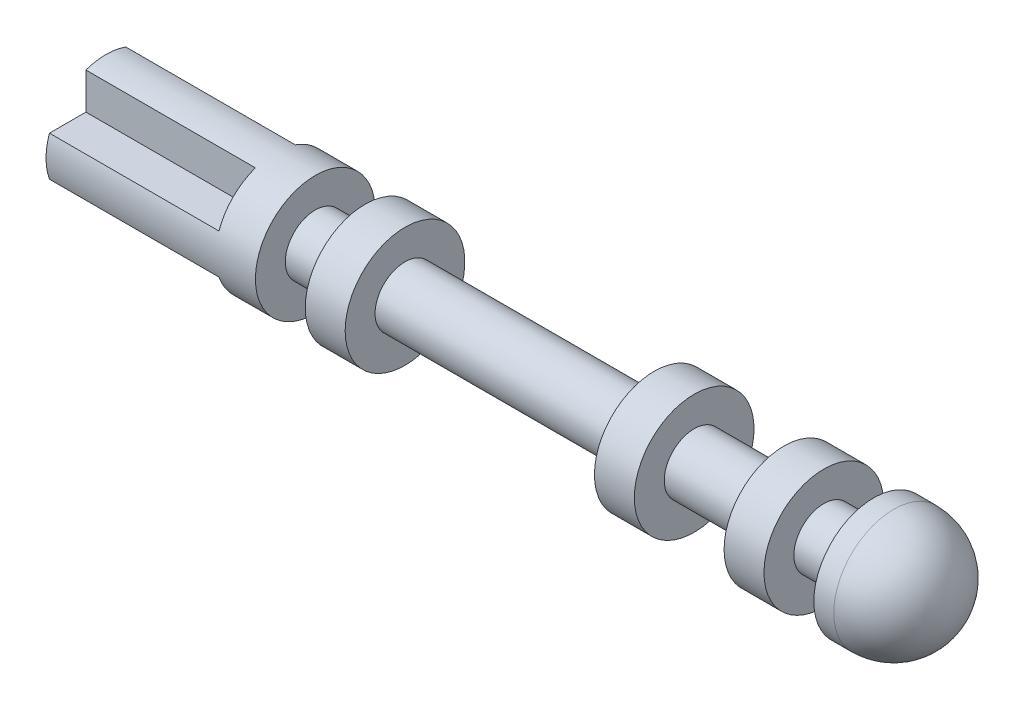
SolidWorks part; units mm, degrees
ref_plane "Front Plane" through (0, 0, 0) normal (0, 0, 1) x (1, 0, 0)
ref_plane "Top Plane" through (0, 0, 0) normal (0, 1, 0) x (1, 0, 0)
ref_plane "Right Plane" through (0, 0, 0) normal (1, 0, 0) x (0, 0, -1)
sketch "Sketch1" plane through (0, 0, 0) normal (0, 0, 1) x (1, 0, 0)
  line L0 (0, 0) -> (141.224, 0) construction
  line L1 (0, 0) -> (0, 3)
  line L2 (0, 3) -> (10.5, 3)
  line L3 (10.5, 3) -> (10.5, 1.5)
  line L4 (10.5, 1.5) -> (13, 1.5)
  line L5 (13, 1.5) -> (13, 3)
  line L6 (13, 3) -> (15, 3)
  line L7 (15, 3) -> (15, 1.5)
  line L8 (15, 1.5) -> (27.5, 1.5)
  line L9 (27.5, 1.5) -> (27.5, 3)
  line L10 (27.5, 3) -> (29.5, 3)
  line L11 (29.5, 3) -> (29.5, 1.5)
  line L12 (29.5, 1.5) -> (34, 1.5)
  line L13 (34, 1.5) -> (34, 3)
  line L14 (34, 3) -> (36, 3)
  line L15 (36, 3) -> (36, 1.5)
  line L16 (36, 1.5) -> (38.5, 1.5)
  line L17 (38.5, 1.5) -> (38.5, 3)
  line L18 (38.5, 3) -> (39.5, 3)
  line L19 (0, 0) -> (42.5, 0)
  arc A0 (39.5, 3) -> (42.5, 0) centre (39.5, 0) cw
  dimension "D5" = 3
  dimension "D1" = 10.5
  dimension "D2" = 2
  dimension "D3" = 2
  dimension "D4" = 2
  dimension "D6" = 39.5
  dimension "D7" = 3
  dimension "D8" = 3
  dimension "D9" = 13
  dimension "D10" = 27.5
  dimension "D11" = 34
  dimension "D12" = 3
  dimension "D13" = 6
  dimension "D14" = 6
  dimension "D15" = 6
  dimension "D16" = 6
  dimension "D17" = 3
  dimension "D18" = 38.5
revolve "Revolve1" add sketch "Sketch1" angle 360 about L0
sketch "Sketch2" plane through (0, 0, 0) normal (-1, 0, 0) x (0, 0, 1)
  line L0 (-4.5005, 1) -> (-4.5005, -1)
  line L1 (-1, -4.5005) -> (1, -4.5005)
  line L2 (-1, -4.5005) -> (-1, 4.5005)
  line L3 (-1, 4.5005) -> (1, 4.5005)
  line L4 (1, -4.5005) -> (1, 4.5005)
  line L5 (-1, -4.5005) -> (1, 4.5005) construction
  line L6 (-1, 4.5005) -> (1, -4.5005) construction
  line L7 (-4.5005, 1) -> (4.5005, 1)
  line L8 (4.5005, 1) -> (4.5005, -1)
  line L9 (-4.5005, -1) -> (4.5005, -1)
  line L10 (-4.5005, 1) -> (4.5005, -1) construction
  line L11 (4.5005, 1) -> (-4.5005, -1) construction
  line L12 (1, 4.5005) -> (-1, 4.5005)
  line L13 (1, 4.5005) -> (1, -4.5005)
  line L14 (1, -4.5005) -> (-1, -4.5005)
  line L15 (-1, 4.5005) -> (-1, -4.5005)
  line L16 (1, 4.5005) -> (-1, -4.5005) construction
  line L17 (1, -4.5005) -> (-1, 4.5005) construction
  line L18 (4.5005, -1) -> (4.5005, 1)
  line L19 (4.5005, -1) -> (-4.5005, -1)
  line L20 (-4.5005, -1) -> (-4.5005, 1)
  line L21 (4.5005, 1) -> (-4.5005, 1)
  line L22 (4.5005, -1) -> (-4.5005, 1) construction
  line L23 (-4.5005, -1) -> (4.5005, 1) construction
  circle A0 centre (0, 0) radius 3
  circle A1 centre (0, 0) radius 3
  circle A2 centre (0, 0) radius 3
  circle A3 centre (0, 0) radius 3
  circle A4 centre (0, 0) radius 3
  point P26 (0, 0)
  circle M1 centre (0, 0) radius 3
  dimension "D2" = 2
  dimension "D3" = 4
  dimension "D1" = 0
extrude "Cut-Extrude1" cut sketch "Sketch2" against normal blind 8.5 contours L4 L7 M1 | L9 L4 M1 | L7 L2 M1 | L9 L2 M1
